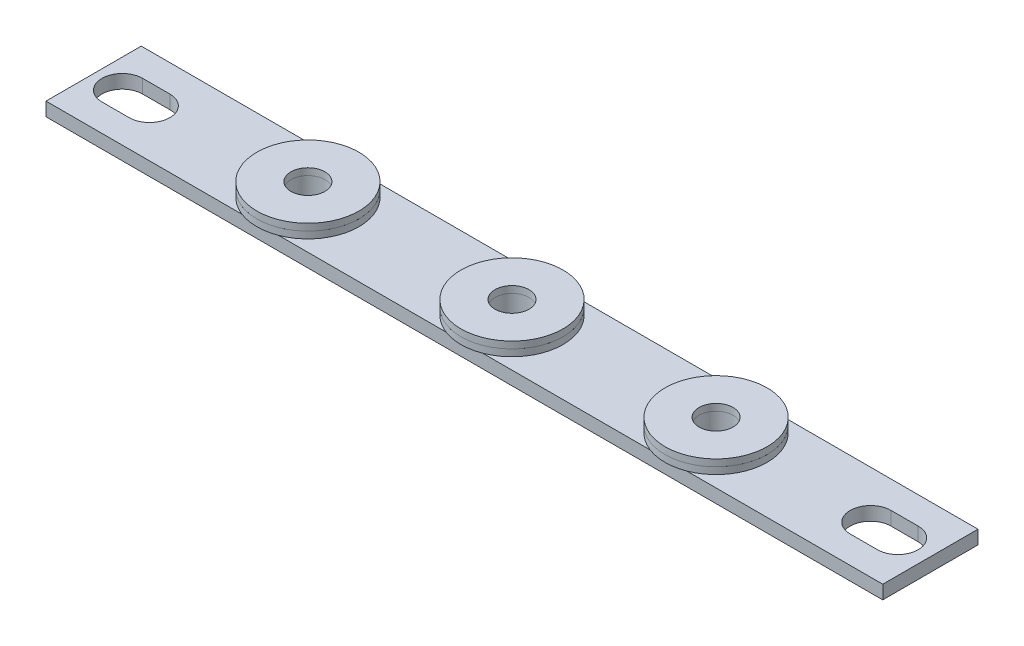
SolidWorks part; units mm, degrees
ref_plane "前视基准面" through (0, 0, 0) normal (0, 0, 1) x (1, 0, 0)
ref_plane "上视基准面" through (0, 0, 0) normal (0, 1, 0) x (1, 0, 0)
ref_plane "右视基准面" through (0, 0, 0) normal (1, 0, 0) x (0, 0, -1)
sketch "草图1" plane through (0, 0, 0) normal (0, 1, 0) x (1, 0, 0)
  line L0 (-57.2857, 0) -> (-53.2857, 0) construction
  line L1 (-61.5, -7) -> (61.5, -7)
  line L2 (-61.5, -7) -> (-61.5, 7)
  line L3 (-61.5, 7) -> (61.5, 7)
  line L4 (61.5, -7) -> (61.5, 7)
  line L5 (-61.5, -7) -> (61.5, 7) construction
  line L6 (-61.5, 7) -> (61.5, -7) construction
  line L7 (-57.2857, 3) -> (-53.2857, 3)
  line L8 (-57.2857, -3) -> (-53.2857, -3)
  line L9 (52.7143, 0) -> (56.7143, 0) construction
  line L10 (52.7143, 3) -> (56.7143, 3)
  line L11 (52.7143, -3) -> (56.7143, -3)
  arc A0 (-57.2857, 3) -> (-57.2857, -3) centre (-57.2857, 0) ccw
  arc A1 (-53.2857, -3) -> (-53.2857, 3) centre (-53.2857, 0) ccw
  arc A2 (52.7143, 3) -> (52.7143, -3) centre (52.7143, 0) ccw
  arc A3 (56.7143, -3) -> (56.7143, 3) centre (56.7143, 0) ccw
  circle A4 centre (-30, 0) radius 2.5
  circle A5 centre (0, 0) radius 2.5
  circle A6 centre (30, 0) radius 2.5
  point P0 (0, 0)
  point P8 (-55.2857, 0)
  point P13 (54.7143, 0)
  dimension "D4" = 3
  dimension "D5" = 3
  dimension "D8" = 5
  dimension "D9" = 5
  dimension "D10" = 5
  dimension "D1" = 123
  dimension "D2" = 14
  dimension "D3" = 110
  dimension "D6" = 4
  dimension "D7" = 4
  dimension "D11" = 30
  dimension "D12" = 30
extrude "凸台-拉伸1" add sketch "草图1" along normal blind 2
sketch "草图2" plane through (0, 2, 0) normal (0, 1, 0) x (1, 0, 0)
  circle A0 centre (-30, 0) radius 2.5
  circle A1 centre (-30, 0) radius 7.5
  circle A2 centre (0, 0) radius 7.5
  circle A3 centre (0, 0) radius 2.5
  circle A4 centre (30, 0) radius 2.5
  circle A5 centre (30, 0) radius 7.5
  dimension "D1" = 15
  dimension "D2" = 15
  dimension "D3" = 15
extrude "凸台-拉伸2" add sketch "草图2" along normal blind 1
sketch "草图3" plane through (0, 3, 0) normal (0, 1, 0) x (1, 0, 0)
  circle A0 centre (-30, 0) radius 2.5
  circle A1 centre (-30, 0) radius 7.5
  circle A2 centre (-30, 0) radius 7.5
  circle A3 centre (0, 0) radius 7.5
  circle A4 centre (0, 0) radius 2.5
  circle A5 centre (30, 0) radius 2.5
  circle A6 centre (30, 0) radius 7.5
  dimension "D2" = 15
  dimension "D3" = 15
  dimension "D1" = 0
extrude "凸台-拉伸3" add sketch "草图3" along normal blind 1 separate body
